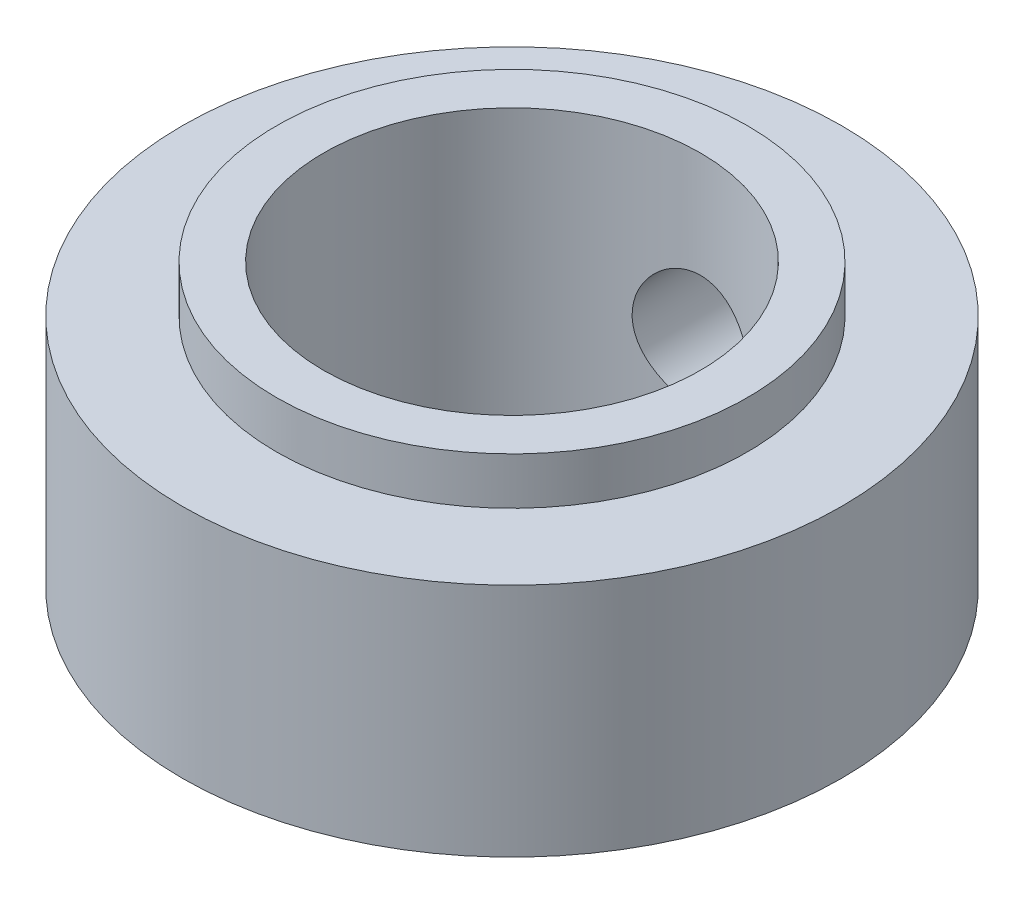
SolidWorks part; units mm, degrees
ref_plane "前视基准面" through (0, 0, 0) normal (0, 0, 1) x (1, 0, 0)
ref_plane "上视基准面" through (0, 0, 0) normal (0, 1, 0) x (1, 0, 0)
ref_plane "右视基准面" through (0, 0, 0) normal (1, 0, 0) x (0, 0, -1)
sketch "草图1" plane through (0, 0, 0) normal (0, 0, 1) x (1, 0, 0)
  line L0 (0, 0) -> (0, 5253.15) construction
  line L1 (4, 4.3683) -> (5, 4.3683)
  line L2 (5, 4.3683) -> (5, 3.3683)
  line L3 (5, 3.3683) -> (7, 3.3683)
  line L4 (7, 3.3683) -> (7, -1.6317)
  line L5 (7, -1.6317) -> (4, -1.6317)
  line L6 (4, -1.6317) -> (4, 4.3683)
  dimension "D1" = 3
  dimension "D2" = 5
  dimension "D3" = 6
  dimension "D4" = 1
  dimension "D5" = 4
revolve "旋转1" add sketch "草图1" angle 360 about L0
sketch "草图2" plane through (0, 0, 0) normal (0, 0, 1) x (1, 0, 0)
  line L0 (-7, -1.6317) -> (7, -1.6317) construction
  circle A0 centre (0, 0.8683) radius 1.25
  dimension "D2" = 2.5
  dimension "D1" = 2.5
extrude "切除-拉伸1" cut sketch "草图2" against normal blind 10
